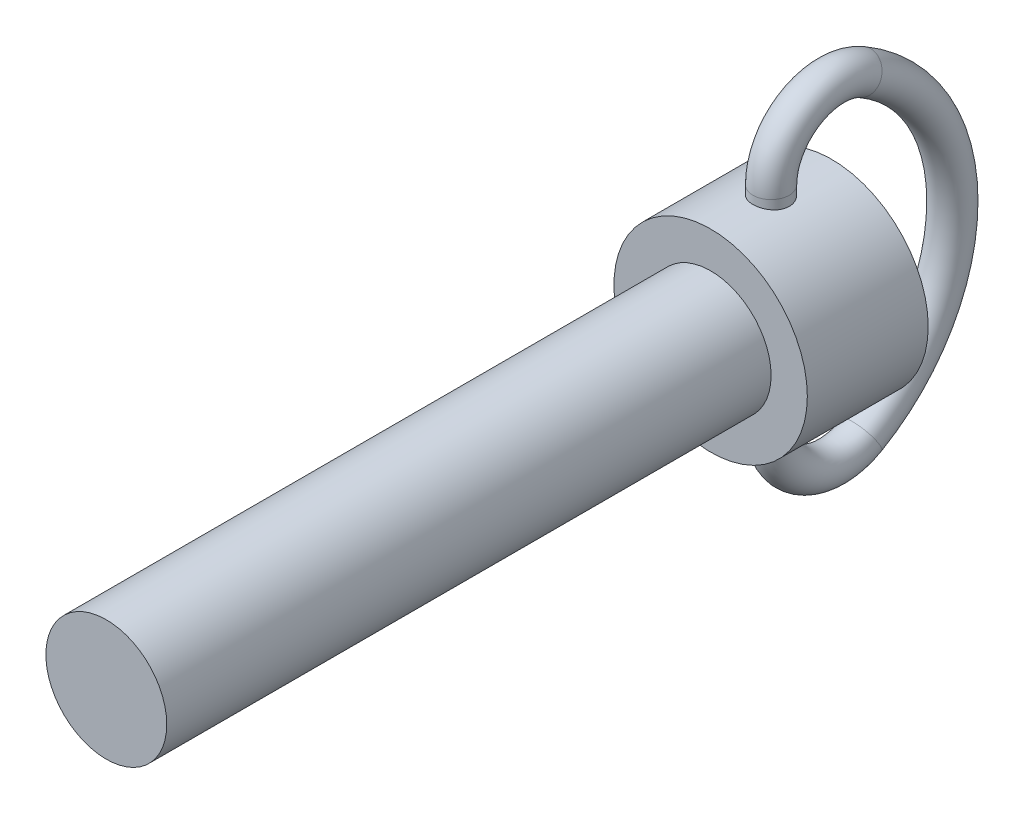
SolidWorks part; units mm, degrees
ref_plane "Front Plane" through (0, 0, 0) normal (0, 0, 1) x (1, 0, 0)
ref_plane "Top Plane" through (0, 0, 0) normal (0, 1, 0) x (1, 0, 0)
ref_plane "Right Plane" through (0, 0, 0) normal (1, 0, 0) x (0, 0, -1)
sketch "Sketch1" plane through (0, 0, 0) normal (0, 0, 1) x (1, 0, 0)
  circle A0 centre (0, 0) radius 4
  dimension "D1" = 8
extrude "Boss-Extrude1" add sketch "Sketch1" along normal blind 5
sketch "Sketch2" plane through (0, 0, 5) normal (0, 0, 1) x (1, 0, 0)
  circle A0 centre (0, 0) radius 2.5
  dimension "D1" = 5
extrude "Boss-Extrude2" add sketch "Sketch2" along normal blind 25
sketch "Sketch3" plane through (0, 0, 0) normal (0, 1, 0) x (1, 0, 0)
  line L0 (0, 0) -> (0, -2.5) construction
  line L1 (0, -2.5) -> (4, -2.5) construction
  line L2 (4, -5) -> (4, 0) construction
  circle A0 centre (0, -2.5) radius 0.75
  dimension "D1" = 1.5
sketch "Sketch4" plane through (0, 0, 0) normal (1, 0, 0) x (0, 0, -1)
  line L0 (-2.5, 0) -> (-2.5, -4.3301)
  line L1 (-1.75, 0) -> (-3.25, 0) construction
  line L2 (-2.5, 4.3301) -> (-2.5, 0)
  arc A0 (1.25, -6.4952) -> (1.25, 6.4952) centre (-2.5, 0) ccw
  arc A1 (1.25, -6.4952) -> (-2.5, -4.3301) centre (0, -4.3301) cw
  arc A2 (1.25, 6.4952) -> (-2.5, 4.3301) centre (0, 4.3301) ccw
  point P8 (-2.5, -7.5)
  dimension "D1" = 7.5
  dimension "D3" = 2.5
  dimension "D2" = 7.5
sweep "Sweep1" add profiles "Sketch3" path "Sketch4"
